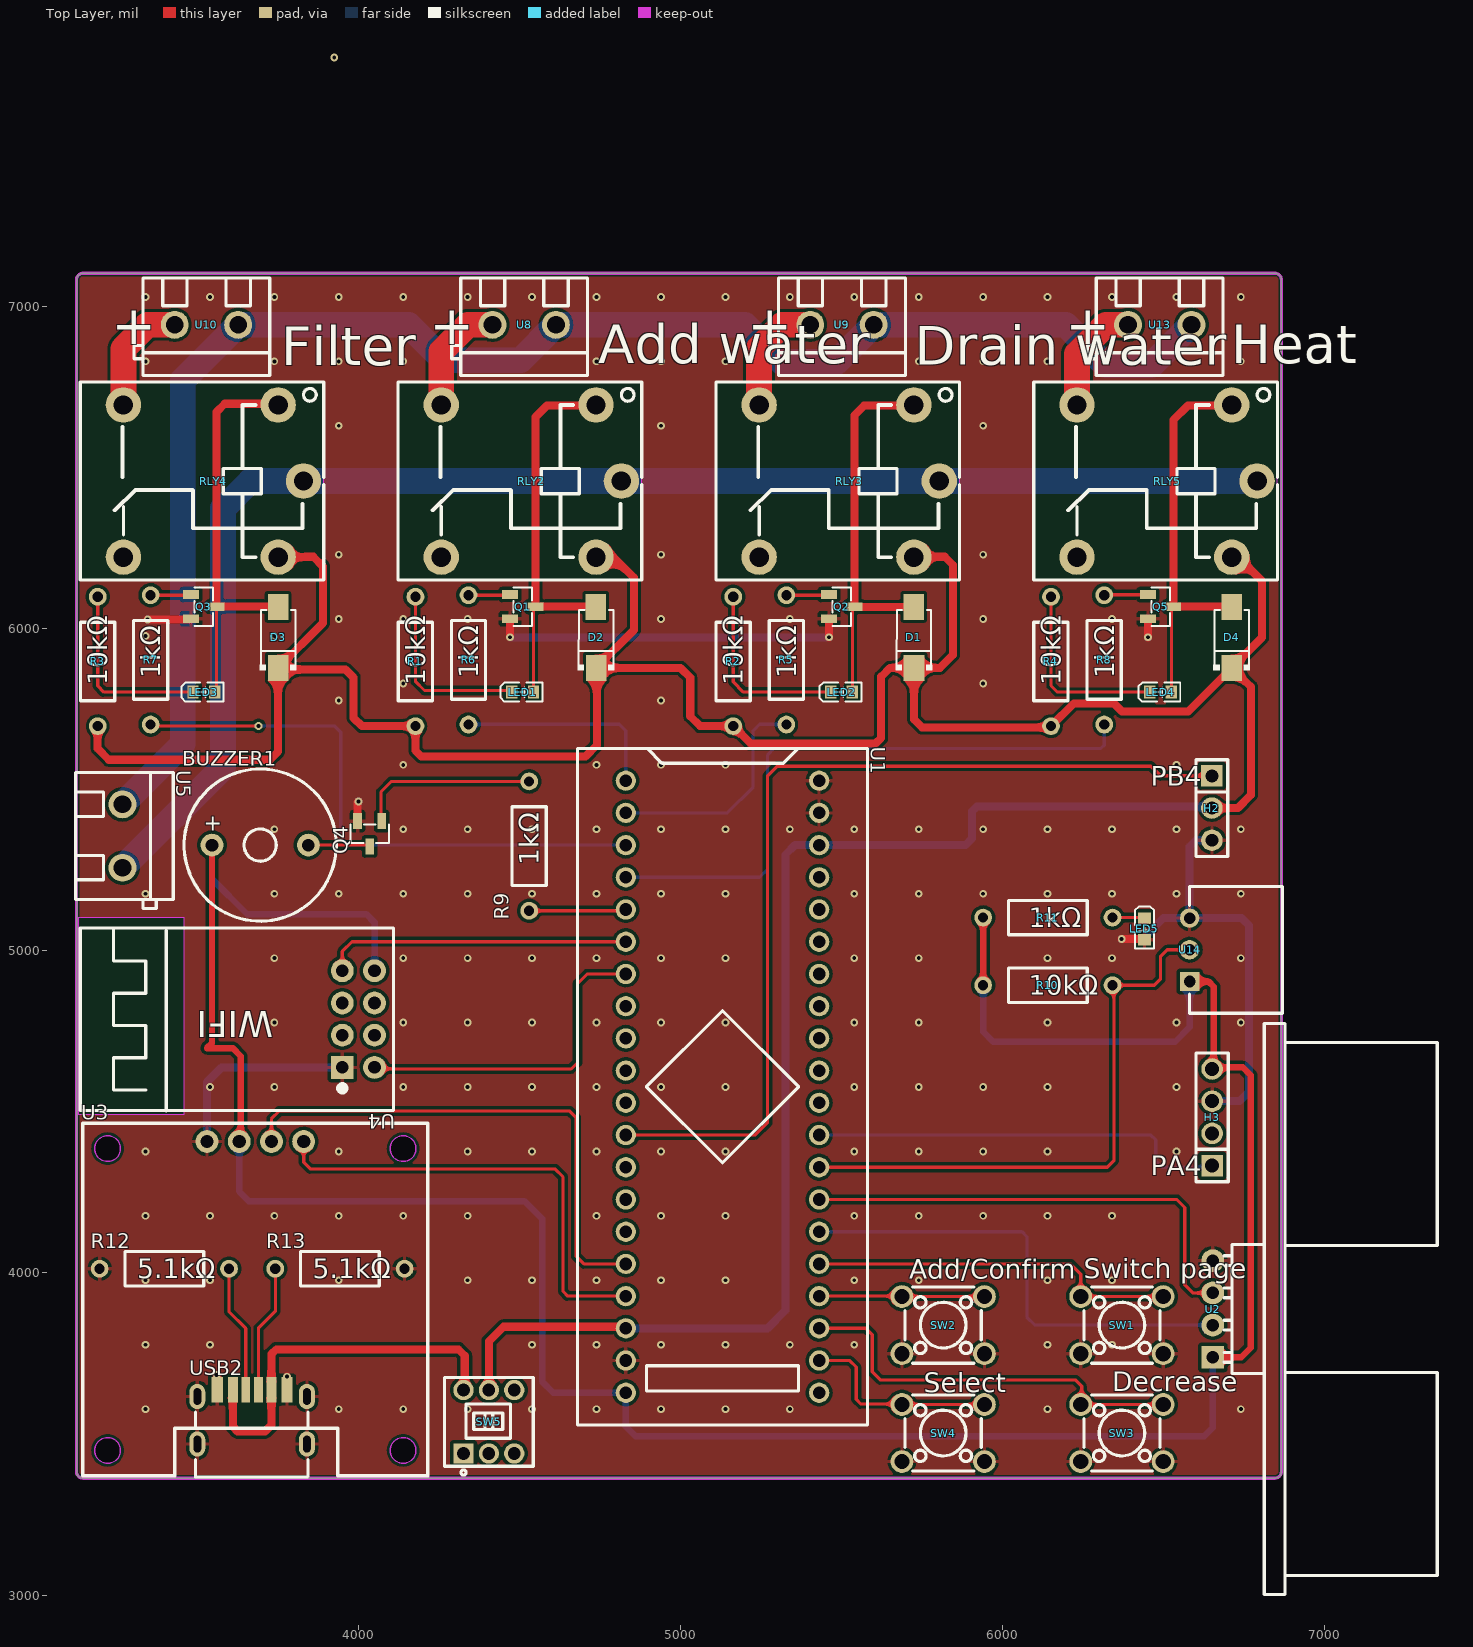
[diagram p0: Top Layer view]
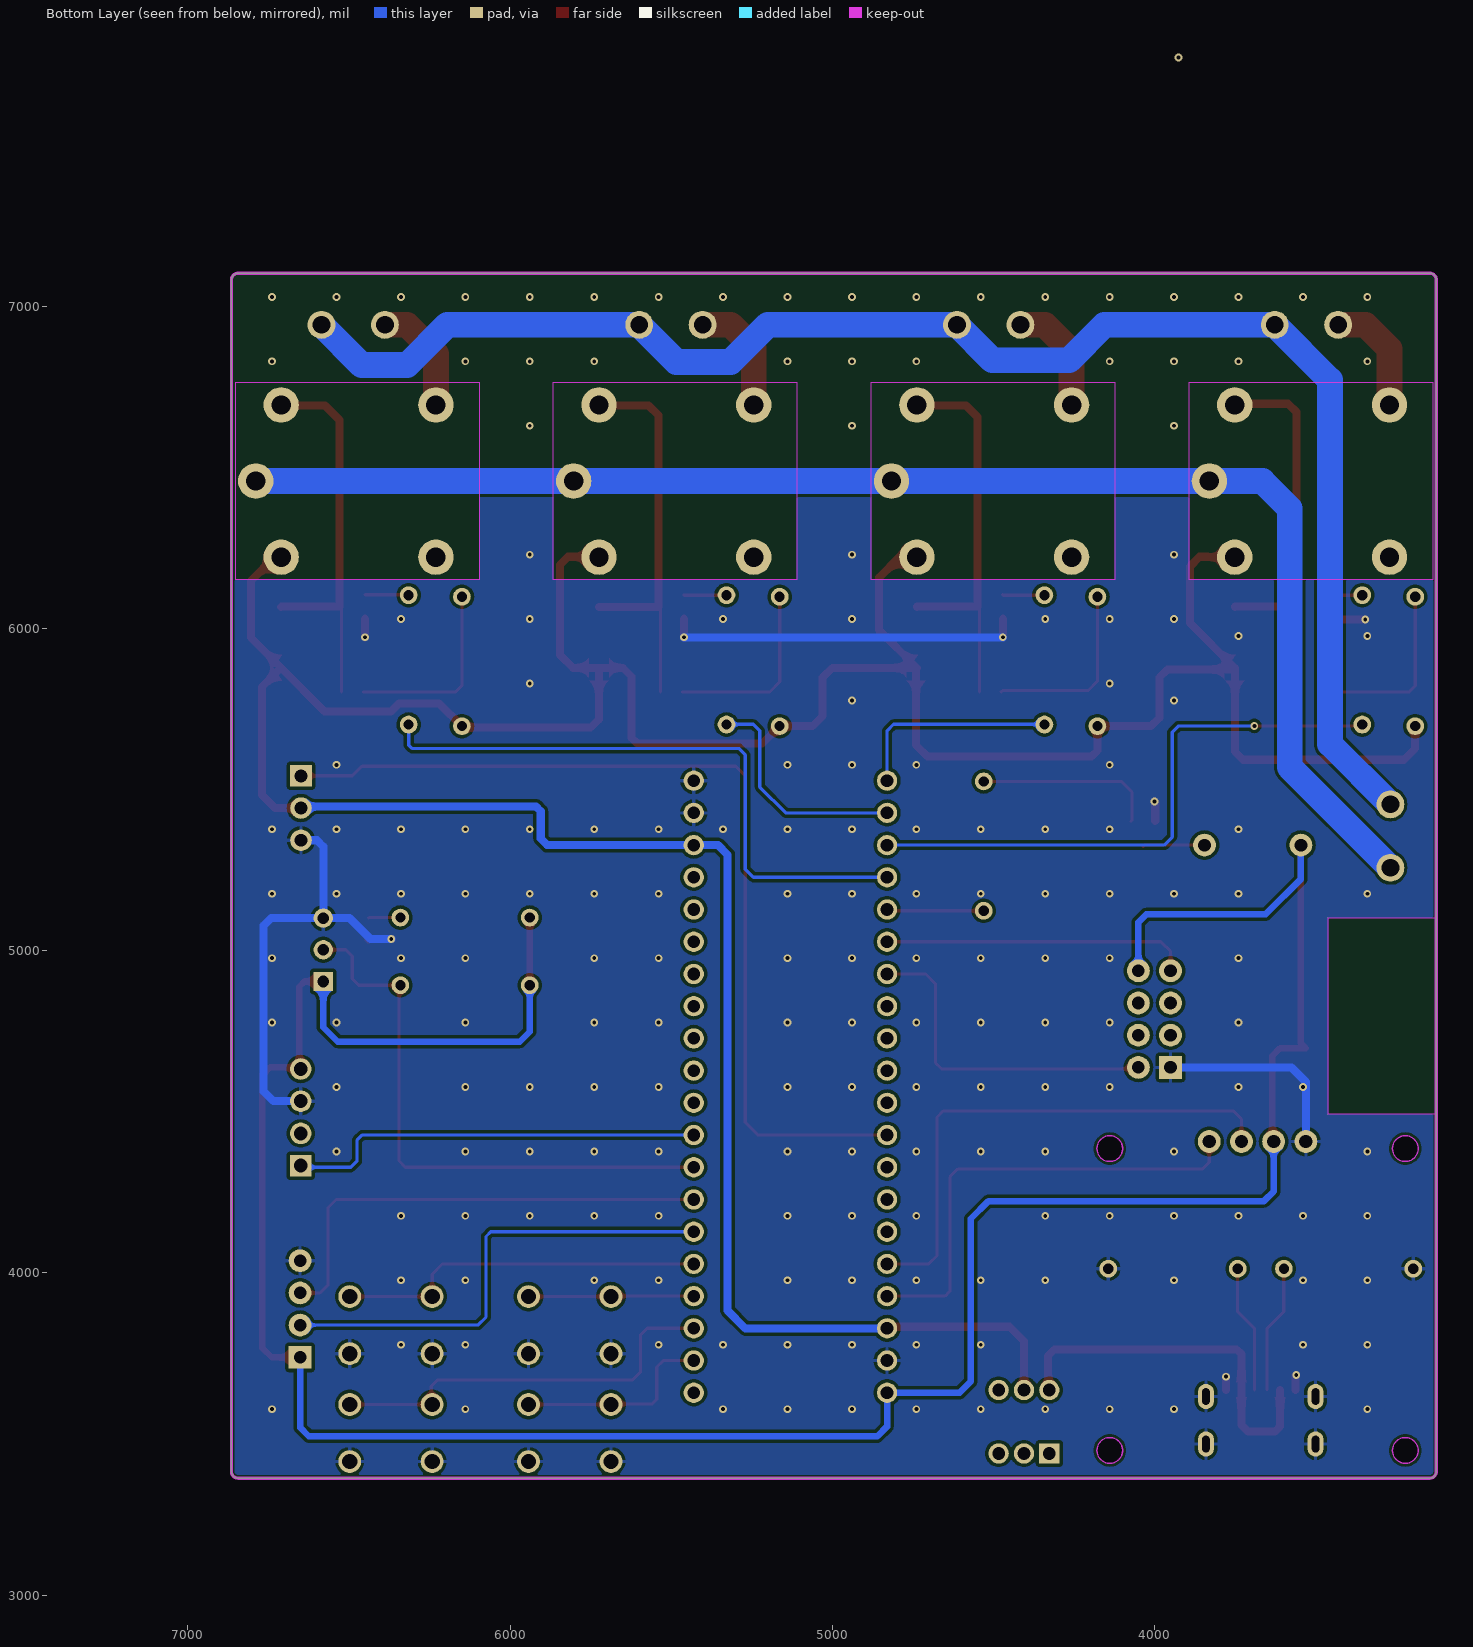
[diagram p1: Bottom Layer view, seen from below]
# Altium PCB MISC62342.pcbdoc (part 1 of 2)
Units mil, origin at the board's own origin, x right, y up, seen from the top; angles counter-clockwise.
Board outline 3740 x 3740 mil, 2 copper layers (Top Layer, Bottom Layer), stack 62.206 mil thick; 50 components, 45 nets, 189 pads, 190 vias.

## Layer stack, top to bottom
Top Solder Mask Layer: solder mask 0.394, Dk 3.3
Top Layer: signal copper 1.379
Dielectric1: surface 59.449, FR4, Dk 4.5
Bottom Layer: signal copper 1.378
Bottom Solder Mask Layer: solder mask 0.394, Dk 3.3

## Board outline
3145,7103.19 ccw(c3145,7083.19) 3125,7083.19 3125,3383.19 ccw(c3145,3383.19) 3145,3363.19 6845,3363.19 ccw(c6845,3383.19) 6865,3383.19 6865,7083.19 ccw(c6845,7083.19) 6845,7103.19

## Design rules (kind name [scope] priority, off if disabled: settings)
BoardOutlineClearance copperThickness2oz_1 [All] p2 off: genericclearance=7.99 ignorepadtopadclearanceinfootprint=FALSE except(0: Arc-SplitContinuation Track-SplitContinuation SMDPad-SplitContinuation THPad-SplitContinuation Via-SplitContinuation Fill-SplitContinuation Region-SplitContinuation Poly-SplitContinuation Text-SplitContinuation Hole-SplitContinuation; 5.98: Arc-CutoutEdge Track-CutoutEdge SMDPad-CutoutEdge THPad-CutoutEdge Via-CutoutEdge Text-CutoutEdge; 6.9: Hole-OutlineEdge Hole-CutoutEdge; 10: Poly-OutlineEdge Poly-CutoutEdge; 11.81: Arc-OutlineEdge Track-OutlineEdge SMDPad-OutlineEdge THPad-OutlineEdge Via-OutlineEdge Fill-OutlineEdge Region-OutlineEdge Text-OutlineEdge Fill-CutoutEdge Region-CutoutEdge)
BoardOutlineClearance Plane_innerPlane_1 [All] p4 off: genericclearance=4.02 ignorepadtopadclearanceinfootprint=FALSE except(0: Arc-SplitContinuation Track-SplitContinuation SMDPad-SplitContinuation THPad-SplitContinuation Via-SplitContinuation Fill-SplitContinuation Region-SplitContinuation Poly-SplitContinuation Text-SplitContinuation Hole-SplitContinuation; 5.98: Arc-CutoutEdge Track-CutoutEdge SMDPad-CutoutEdge THPad-CutoutEdge Via-CutoutEdge Text-CutoutEdge; 6.9: Hole-OutlineEdge Hole-CutoutEdge; 10: Poly-OutlineEdge Poly-CutoutEdge; 11.81: Arc-OutlineEdge Track-OutlineEdge SMDPad-OutlineEdge THPad-OutlineEdge Via-OutlineEdge Fill-OutlineEdge Region-OutlineEdge Text-OutlineEdge Fill-CutoutEdge Region-CutoutEdge)
BoardOutlineClearance Copper_copperRegion_1 [All] p6 off: genericclearance=4.02 ignorepadtopadclearanceinfootprint=FALSE except(0: Arc-SplitContinuation Track-SplitContinuation SMDPad-SplitContinuation THPad-SplitContinuation Via-SplitContinuation Fill-SplitContinuation Region-SplitContinuation Poly-SplitContinuation Text-SplitContinuation Hole-SplitContinuation; 5.98: Arc-CutoutEdge Track-CutoutEdge SMDPad-CutoutEdge THPad-CutoutEdge Via-CutoutEdge Text-CutoutEdge; 6.9: Hole-OutlineEdge Hole-CutoutEdge; 10: Poly-OutlineEdge Poly-CutoutEdge; 11.81: Arc-OutlineEdge Track-OutlineEdge SMDPad-OutlineEdge THPad-OutlineEdge Via-OutlineEdge Fill-OutlineEdge Region-OutlineEdge Text-OutlineEdge Fill-CutoutEdge Region-CutoutEdge)
BoardOutlineClearance copperThickness1oz_1 [All] p8: genericclearance=4.02 ignorepadtopadclearanceinfootprint=FALSE except(0: Arc-SplitContinuation Track-SplitContinuation SMDPad-SplitContinuation THPad-SplitContinuation Via-SplitContinuation Fill-SplitContinuation Region-SplitContinuation Poly-SplitContinuation Text-SplitContinuation Hole-SplitContinuation; 5.98: Arc-CutoutEdge Track-CutoutEdge SMDPad-CutoutEdge THPad-CutoutEdge Via-CutoutEdge Text-CutoutEdge; 6.9: Hole-OutlineEdge Hole-CutoutEdge; 10: Poly-OutlineEdge Poly-CutoutEdge; 11.81: Arc-OutlineEdge Track-OutlineEdge SMDPad-OutlineEdge THPad-OutlineEdge Via-OutlineEdge Fill-OutlineEdge Region-OutlineEdge Text-OutlineEdge Fill-CutoutEdge Region-CutoutEdge)
Clearance copperThickness2oz [All] p1 off: gap=7.99 ignorepadtopadclearanceinfootprint=FALSE except(5.98: SMDPad-Track SMDPad-SMDPad THPad-Track SMDPad-THPad THPad-THPad Track-Via SMDPad-Via THPad-Via Via-Via Fill-SMDPad Region-SMDPad Fill-THPad Region-THPad Fill-Via Region-Via Fill-Fill Fill-Region Region-Region Arc-Track Arc-SMDPad Arc-THPad Arc-Via Fill-Arc Region-Arc Arc-Arc Text-Track SMDPad-Text Text-THPad Text-Via Fill-Text Region-Text Arc-Text Text-Text; 6.9: Hole-Track Hole-SMDPad Hole-THPad Hole-Via Fill-Hole Region-Hole Hole-Arc Hole-Text; 10: Poly-Track Poly-SMDPad Poly-THPad Poly-Via Poly-Fill Poly-Region Poly-Poly Poly-Arc Poly-Text Poly-Hole; 11.81: Fill-Track Region-Track)
Clearance Plane_innerPlane [All] p3 off: gap=4.02 ignorepadtopadclearanceinfootprint=FALSE except(5.98: SMDPad-Track SMDPad-SMDPad THPad-Track SMDPad-THPad THPad-THPad Track-Via SMDPad-Via THPad-Via Via-Via Fill-SMDPad Region-SMDPad Fill-THPad Region-THPad Fill-Via Region-Via Fill-Fill Fill-Region Region-Region Arc-Track Arc-SMDPad Arc-THPad Arc-Via Fill-Arc Region-Arc Arc-Arc Text-Track SMDPad-Text Text-THPad Text-Via Fill-Text Region-Text Arc-Text Text-Text; 6.9: Hole-Track Hole-SMDPad Hole-THPad Hole-Via Fill-Hole Region-Hole Hole-Arc Hole-Text; 10: Poly-Track Poly-SMDPad Poly-THPad Poly-Via Poly-Fill Poly-Region Poly-Poly Poly-Arc Poly-Text Poly-Hole; 11.81: Fill-Track Region-Track)
Clearance Copper_copperRegion [All] p5 off: gap=4.02 ignorepadtopadclearanceinfootprint=FALSE except(5.98: SMDPad-Track SMDPad-SMDPad THPad-Track SMDPad-THPad THPad-THPad Track-Via SMDPad-Via THPad-Via Via-Via Fill-SMDPad Region-SMDPad Fill-THPad Region-THPad Fill-Via Region-Via Fill-Fill Fill-Region Region-Region Arc-Track Arc-SMDPad Arc-THPad Arc-Via Fill-Arc Region-Arc Arc-Arc Text-Track SMDPad-Text Text-THPad Text-Via Fill-Text Region-Text Arc-Text Text-Text; 6.9: Hole-Track Hole-SMDPad Hole-THPad Hole-Via Fill-Hole Region-Hole Hole-Arc Hole-Text; 10: Poly-Track Poly-SMDPad Poly-THPad Poly-Via Poly-Fill Poly-Region Poly-Poly Poly-Arc Poly-Text Poly-Hole; 11.81: Fill-Track Region-Track)
Clearance copperThickness1oz [All] p7: gap=4.02 ignorepadtopadclearanceinfootprint=FALSE except(5.98: SMDPad-Track SMDPad-SMDPad THPad-Track SMDPad-THPad THPad-THPad Track-Via SMDPad-Via THPad-Via Via-Via Fill-SMDPad Region-SMDPad Fill-THPad Region-THPad Fill-Via Region-Via Fill-Fill Fill-Region Region-Region Arc-Track Arc-SMDPad Arc-THPad Arc-Via Fill-Arc Region-Arc Arc-Arc Text-Track SMDPad-Text Text-THPad Text-Via Fill-Text Region-Text Arc-Text Text-Text; 6.9: Hole-Track Hole-SMDPad Hole-THPad Hole-Via Fill-Hole Region-Hole Hole-Arc Hole-Text; 10: Poly-Track Poly-SMDPad Poly-THPad Poly-Via Poly-Fill Poly-Region Poly-Poly Poly-Arc Poly-Text Poly-Hole; 11.81: Fill-Track Region-Track)
DiffPairsRouting differentialPair [All] p1: maxlimit=6 minlimit=6 mostfreqgap=6 toplayer_minwidth=5 toplayer_prefwidth=10 toplayer_maxwidth=100 toplayer_mingap=6 toplayer_prefgap=6 toplayer_maxgap=6 bottomlayer_minwidth=5 bottomlayer_prefwidth=10 bottomlayer_maxwidth=100 bottomlayer_mingap=6 bottomlayer_prefgap=6 bottomlayer_maxgap=6 maxuncoupledlength=10
HoleToHoleClearance otherClearance [All] p1: gap=11.81 allowstackedmicrovias=TRUE
Length netLength [All] p1: minlimit=0 maxlimit=0
PasteMaskExpansion pasteMaskExpansion [All] p1: expansion=0
PlaneConnect innerPlane [All] p1: planeconnectstyle=Relief reliefexpansion=20 reliefentries=4 reliefconductorwidth=10 reliefairgap=10
PolygonConnect copperRegion [All] p1: connectstyle=Relief reliefconductorwidth=10 reliefentries=4 polygonreliefangle="90 Angle" airgapwidth=10 via.connectstyle=Relief via.reliefconductorwidth=10 via.reliefentries=4 via.polygonreliefangle="90 Angle" via.airgapwidth=10
RoutingVias viaSize [All] p1: holewidth=12.01 width=24.02 viastyle="Through Hole" minholewidth=11.81 minwidth=19.68 maxholewidth=248.03 maxwidth=393.7
SolderMaskExpansion solderMaskExpansion [IsVia] p1: expansion=-1000 istentingtop=TRUE
SolderMaskExpansion solderMaskExpansion [All] p2: expansion=2 istentingtop=FALSE
Width copperThickness2oz_2 [All] p1 off: maxlimit=100 minlimit=8 preferedwidth=10
Width copperThickness1oz_2 [All] p2: maxlimit=100 minlimit=5 preferedwidth=10

## Components (designator, comment, footprint, x,y, rotation, side; value= is the part's Value field where it differs from the comment)
BUZZER1 "2.4kHz" BUZ-TH_BD12.0-P7.60-D0.6-FD 3695,5328.19 r0 top
D1 "1N4007A-AAF" SMA_L4.3-W2.6-LS5.0-RD 5724.12,5973.19 r90 top
D2 "1N4007A-AAF" SMA_L4.3-W2.6-LS5.0-RD 4737.46,5973.19 r90 top
D3 "1N4007A-AAF" SMA_L4.3-W2.6-LS5.0-RD 3750.79,5973.19 r90 top
D4 "1N4007A-AAF" SMA_L4.3-W2.6-LS5.0-RD 6710.79,5973.19 r90 top
H2 "PZ254V-11-03P" HDR-TH_3P-P2.54-V-M_PZ254V-11-03P 6649.21,5443.19 r270 top
H3 "PZ254V-11-04P" HDR-TH_4P-P2.54-V-M 6650,4483.19 r90 top
LED1 "GL0603UR01" LED0603-FD 4510,5803.19 r180 top
LED2 "GL0603UR01" LED0603-FD 5500,5803.19 r180 top
LED3 "GL0603UR01" LED0603-FD 3520,5803.19 r180 top
LED4 "GL0603UR01" LED0603-FD 6490,5803.19 r180 top
LED5 "GL0603UR01" LED0603-FD 6440,5068.19 r90 top
Q1 "SS8050" SOT-23-3_L2.9-W1.3-P1.90-LS2.4-BR 4510,6068.19 r180 top
Q2 "SS8050" SOT-23-3_L2.9-W1.3-P1.90-LS2.4-BR 5500,6068.19 r180 top
Q3 "SS8050" SOT-23-3_L2.9-W1.3-P1.90-LS2.4-BR 3520,6068.19 r180 top
Q4 "SS8050" SOT-23-3_L2.9-W1.3-P1.90-LS2.4-BR 4035,5363.19 r90 top
Q5 "SS8050" SOT-23-3_L2.9-W1.3-P1.90-LS2.4-BR 6490,6068.19 r180 top
R1 "10kΩ" RES-TH_BD2.7-L6.2-P10.20-D0.4 4177.02,5898.19 r270 top
R2 "10kΩ" RES-TH_BD2.7-L6.2-P10.20-D0.4 5163.37,5898.19 r270 top
R3 "10kΩ" RES-TH_BD2.7-L6.2-P10.20-D0.4 3190.66,5898.19 r270 top
R4 "10kΩ" RES-TH_BD2.7-L6.2-P10.20-D0.4 6149.72,5898.19 r270 top
R5 "1kΩ" RES-TH_BD2.7-L6.2-P10.20-D0.4 5328.33,5903.19 r90 top
R6 "1kΩ" RES-TH_BD2.7-L6.2-P10.20-D0.4 4341.67,5903.19 r90 top
R7 "1kΩ" RES-TH_BD2.7-L6.2-P10.20-D0.4 3355,5903.19 r90 top
R8 "1kΩ" RES-TH_BD2.7-L6.2-P10.20-D0.4 6315,5903.19 r90 top
R9 "1kΩ" RES-TH_BD2.7-L6.2-P10.20-D0.4 4530,5325.04 r90 top
R10 "10kΩ" RES-TH_BD2.7-L6.2-P10.20-D0.4 6140,4893.19 r180 top
R11 "1kΩ" RES-TH_BD2.7-L6.2-P10.20-D0.4 6140,5103.19 r180 top
R12 "5.1kΩ" RES-TH_BD2.7-L6.2-P10.20-D0.4 3397.56,4013.19 r0 top
R13 "5.1kΩ" RES-TH_BD2.7-L6.2-P10.20-D0.4 3942.44,4013.19 r0 top
RLY2 "SRD-05VDC-SL-C" RELAY-TH_SRD-XXVDC-XL-C 4536.67,6458.19 r180 top
RLY3 "SRD-05VDC-SL-C" RELAY-TH_SRD-XXVDC-XL-C 5523.33,6458.19 r180 top
RLY4 "SRD-05VDC-SL-C" RELAY-TH_SRD-XXVDC-XL-C 3550,6458.19 r180 top
RLY5 "SRD-05VDC-SL-C" RELAY-TH_SRD-XXVDC-XL-C 6510,6458.19 r180 top
SW1 "TS665CJ" SW-TH_4P-L6.0-W6.0-P4.50-LS6.5 6370,3838.19 r0 top
SW2 "TS665CJ" SW-TH_4P-L6.0-W6.0-P4.50-LS6.5 5815,3838.19 r0 top
SW3 "TS665CJ" SW-TH_4P-L6.0-W6.0-P4.50-LS6.5 6370,3503.19 r0 top
SW4 "TS665CJ" SW-TH_4P-L6.0-W6.0-P4.50-LS6.5 5815,3503.19 r0 top
SW5 "TK-6700-1" SW-TH_TK-6700-1 4405,3538.19 r0 top
U1 "LCKFB-DKX-STM32F103C8T6" CONN-TH_L53.3-W22.9_STM32F103C8T6-CARD 5130,4578.19 r270 top
U2 "HC-SR04" TH_HC-SR04V 6651.97,3888.19 r90 top
U3 "HS96L03W2C03" OLED-TH_L27.8-W27.2-P2.54_C9900033791 3680,4408.19 r0 top
U4 "2.4GHz" WIFIM-TH_8P-L24.7-W14.4-P2.54 4000,4788.19 r180 top
U5 "KF301-5.0-2P" CONN-TH_P5.00_KF301-5.0-2P 3267.64,5356.28 r270 top
U8 "KF301-5.0-2P" CONN-TH_P5.00_KF301-5.0-2P 4514.53,6943.19 r180 top
U9 "KF301-5.0-2P" CONN-TH_P5.00_KF301-5.0-2P 5500.88,6943.19 r180 top
U10 "KF301-5.0-2P" CONN-TH_P5.00_KF301-5.0-2P 3528.18,6943.19 r180 top
U13 "KF301-5.0-2P" CONN-TH_P5.00_KF301-5.0-2P 6487.23,6943.19 r180 top
U14 "WAFER-XH2.54-3PWZ" CONN-TH_3P-P2.50_WAFER-XH2.54-3PWZ 6580,5003.19 r90 top
USB2 "" "USB_ TYPE-C-6P" 3665,3553.19 r0 top

## Footprints (in the part's own frame and the unit in brackets; to place one, negate y for a bottom-side part, rotate by r counter-clockwise, add the part's x,y. Pads: shape width x height; smd on the part's side, far side on the other; paste and mask are expansions set on the pad)
BUZ-TH_BD12.0-P7.60-D0.6-FD [mm]
  round 1.8 hole 1: 1(-3.8,0) 2(3.8,0)
  silkscreen extent -6,-6 6,6
CONN-TH_3P-P2.50_WAFER-XH2.54-3PWZ [mil]
  rect 60x60 hole 36 paste+0 mask+1.97: 1(-98.43,0)
  round 60 hole 36 paste+0 mask+1.97: 2(-0.01,0) 3(98.42,0)
  silkscreen extent -197,-288 197,0
CONN-TH_L53.3-W22.9_STM32F103C8T6-CARD [mm]
  round 1.6 hole 1: 1(-24.13,-7.62) 2(-21.59,-7.62) 3(-19.05,-7.62) 4(-16.51,-7.62) 5(-13.97,-7.62) 6(-11.43,-7.62) 7(-8.89,-7.62) 8(-6.35,-7.62) 9(-3.81,-7.62) 10(-1.27,-7.62) 11(1.27,-7.62) 12(3.81,-7.62) 13(6.35,-7.62) 14(8.89,-7.62) 15(11.43,-7.62) 16(13.97,-7.62) 17(16.51,-7.62) 18(19.05,-7.62) 19(21.59,-7.62) 20(24.13,-7.62) 21(24.13,7.62) 22(21.59,7.62) 23(19.05,7.62) 24(16.51,7.62) 25(13.97,7.62) 26(11.43,7.62) 27(8.89,7.62) 28(6.35,7.62) 29(3.81,7.62) 30(1.27,7.62) 31(-1.27,7.62) 32(-3.81,7.62) 33(-6.35,7.62) 34(-8.89,7.62) 35(-11.43,7.62) 36(-13.97,7.62) 37(-16.51,7.62) 38(-19.05,7.62) 39(-21.59,7.62) 40(-24.13,7.62)
  silkscreen extent -26.67,-11.43 26.67,11.43
CONN-TH_P5.00_KF301-5.0-2P [mm]
  round 2.2 hole 1.4 paste+0 mask+0.05: 1(-2.5,0) 2(2.5,0)
  silkscreen extent -5,-3.7 5.71,4
HDR-TH_3P-P2.54-V-M_PZ254V-11-03P [mm]
  rect 1.7x1.7 hole 1.02: 1(-2.54,0)
  round 1.7 hole 1.02: 2(0,0) 3(2.54,0)
  silkscreen extent -3.81,-1.25 3.81,1.25
HDR-TH_4P-P2.54-V-M [mm]
  rect 1.7x1.7 hole 1.1: 1(-3.81,0)
  round 1.7 hole 1.1: 2(-1.27,0) 3(1.27,0) 4(3.81,0)
  silkscreen extent -5.08,-1.27 5.08,1.27
LED0603-FD [mm]
  rect 0.9x1 smd: 1(-0.85,0) 2(0.85,0)
  silkscreen extent -1.55,-0.75 1.75,0.75
OLED-TH_L27.8-W27.2-P2.54_C9900033791 [mm]
  round 1.8 hole 1.05 paste+0 mask+0.05: 1(-3.81,0) 2(-1.27,0) 3(1.27,0) 4(3.81,0)
  Board Outline Layer circle w0.003: c-11.65,-0.56 r1.016
  Board Outline Layer circle w0.003: c11.65,-0.56 r1.016
  Board Outline Layer circle w0.003: c-11.65,-24.36 r1.016
  Board Outline Layer circle w0.003: c11.65,-24.36 r1.016
  Board Outline Layer region: -10.634,-0.56 -10.735,-1.001 -11.016,-1.354 -11.424,-1.551 -11.876,-1.551 -12.283,-1.354 -12.565,-1.001 -12.666,-0.56 -12.666,-0.56 -12.565,-0.119 -12.283,0.234 -11.876,0.431 -11.424,0.431 -11.016,0.234 -10.735,-0.119 -10.634,-0.56
  Board Outline Layer region: -10.634,-0.56 -10.643,-0.698 -10.672,-0.834 -10.718,-0.965 -10.782,-1.088 -10.862,-1.201 -10.956,-1.303 -11.064,-1.39 -11.183,-1.462 -11.31,-1.517 -11.443,-1.555 -11.581,-1.574 -11.719,-1.574 -11.857,-1.555 -11.99,-1.517 -12.117,-1.462 -12.236,-1.39 -12.343,-1.303 -12.438,-1.201 -12.518,-1.088 -12.582,-0.965 -12.628,-0.834 -12.656,-0.698 -12.666,-0.56 -12.656,-0.422 -12.628,-0.286 -12.582,-0.155 -12.518,-0.032 -12.438,0.081 -12.343,0.183 -12.236,0.27 -12.117,0.342 -11.99,0.397 -11.857,0.435 -11.719,0.454 -11.581,0.454 -11.443,0.435 -11.31,0.397 -11.183,0.342 -11.064,0.27 -10.956,0.183 -10.862,0.081 -10.782,-0.032 -10.718,-0.155 -10.672,-0.286 -10.643,-0.422
  Board Outline Layer region: 12.666,-0.56 12.565,-1.001 12.283,-1.354 11.876,-1.551 11.424,-1.551 11.017,-1.354 10.735,-1.001 10.634,-0.56 10.634,-0.56 10.735,-0.119 11.017,0.234 11.424,0.431 11.876,0.431 12.283,0.234 12.565,-0.119 12.666,-0.56
  Board Outline Layer region: 12.666,-0.56 12.657,-0.698 12.628,-0.834 12.582,-0.965 12.518,-1.088 12.438,-1.201 12.343,-1.303 12.236,-1.39 12.117,-1.462 11.99,-1.517 11.857,-1.555 11.719,-1.574 11.581,-1.574 11.443,-1.555 11.31,-1.517 11.183,-1.462 11.064,-1.39 10.957,-1.303 10.862,-1.201 10.782,-1.088 10.718,-0.965 10.672,-0.834 10.643,-0.698 10.634,-0.56 10.643,-0.422 10.672,-0.286 10.718,-0.155 10.782,-0.032 10.862,0.081 10.957,0.183 11.064,0.27 11.183,0.342 11.31,0.397 11.443,0.435 11.581,0.454 11.719,0.454 11.857,0.435 11.99,0.397 12.117,0.342 12.236,0.27 12.343,0.183 12.438,0.081 12.518,-0.032 12.582,-0.155 12.628,-0.286 12.657,-0.422
  Board Outline Layer region: -10.634,-24.36 -10.735,-24.801 -11.016,-25.154 -11.424,-25.35 -11.876,-25.35 -12.283,-25.154 -12.565,-24.801 -12.666,-24.36 -12.666,-24.36 -12.565,-23.919 -12.283,-23.566 -11.876,-23.369 -11.424,-23.369 -11.016,-23.566 -10.735,-23.919 -10.634,-24.36
  Board Outline Layer region: -10.634,-24.36 -10.643,-24.498 -10.672,-24.634 -10.718,-24.765 -10.782,-24.888 -10.862,-25.001 -10.956,-25.102 -11.064,-25.19 -11.183,-25.262 -11.31,-25.317 -11.443,-25.355 -11.581,-25.374 -11.719,-25.374 -11.857,-25.355 -11.99,-25.317 -12.117,-25.262 -12.236,-25.19 -12.343,-25.102 -12.438,-25.001 -12.518,-24.888 -12.582,-24.765 -12.628,-24.634 -12.656,-24.498 -12.666,-24.36 -12.656,-24.222 -12.628,-24.086 -12.582,-23.955 -12.518,-23.832 -12.438,-23.719 -12.343,-23.617 -12.236,-23.53 -12.117,-23.458 -11.99,-23.403 -11.857,-23.365 -11.719,-23.346 -11.581,-23.346 -11.443,-23.365 -11.31,-23.403 -11.183,-23.458 -11.064,-23.53 -10.956,-23.617 -10.862,-23.719 -10.782,-23.832 -10.718,-23.955 -10.672,-24.086 -10.643,-24.222
  Board Outline Layer region: 12.666,-24.36 12.565,-24.801 12.283,-25.154 11.876,-25.35 11.424,-25.35 11.017,-25.154 10.735,-24.801 10.634,-24.36 10.634,-24.36 10.735,-23.919 11.017,-23.566 11.424,-23.369 11.876,-23.369 12.283,-23.566 12.565,-23.919 12.666,-24.36
  Board Outline Layer region: 12.666,-24.36 12.657,-24.498 12.628,-24.634 12.582,-24.765 12.518,-24.888 12.438,-25.001 12.343,-25.102 12.236,-25.19 12.117,-25.262 11.99,-25.317 11.857,-25.355 11.719,-25.374 11.581,-25.374 11.443,-25.355 11.31,-25.317 11.183,-25.262 11.064,-25.19 10.957,-25.102 10.862,-25.001 10.782,-24.888 10.718,-24.765 10.672,-24.634 10.643,-24.498 10.634,-24.36 10.643,-24.222 10.672,-24.086 10.718,-23.955 10.782,-23.832 10.862,-23.719 10.957,-23.617 11.064,-23.53 11.183,-23.458 11.31,-23.403 11.443,-23.365 11.581,-23.346 11.719,-23.346 11.857,-23.365 11.99,-23.403 12.117,-23.458 12.236,-23.53 12.343,-23.617 12.438,-23.719 12.518,-23.832 12.582,-23.955 12.628,-24.086 12.657,-24.222
  Multi-Layer board cut-out: -10.634,-0.56 -10.735,-1.001 -11.016,-1.354 -11.424,-1.551 -11.876,-1.551 -12.283,-1.354 -12.565,-1.001 -12.666,-0.56 -12.666,-0.56 -12.565,-0.119 -12.283,0.234 -11.876,0.431 -11.424,0.431 -11.016,0.234 -10.735,-0.119 -10.634,-0.56
  Multi-Layer board cut-out: 12.666,-0.56 12.565,-1.001 12.283,-1.354 11.876,-1.551 11.424,-1.551 11.017,-1.354 10.735,-1.001 10.634,-0.56 10.634,-0.56 10.735,-0.119 11.017,0.234 11.424,0.431 11.876,0.431 12.283,0.234 12.565,-0.119 12.666,-0.56
  Multi-Layer board cut-out: -10.634,-24.36 -10.735,-24.801 -11.016,-25.154 -11.424,-25.35 -11.876,-25.35 -12.283,-25.154 -12.565,-24.801 -12.666,-24.36 -12.666,-24.36 -12.565,-23.919 -12.283,-23.566 -11.876,-23.369 -11.424,-23.369 -11.016,-23.566 -10.735,-23.919 -10.634,-24.36
  Multi-Layer board cut-out: 12.666,-24.36 12.565,-24.801 12.283,-25.154 11.876,-25.35 11.424,-25.35 11.017,-25.154 10.735,-24.801 10.634,-24.36 10.634,-24.36 10.735,-23.919 11.017,-23.566 11.424,-23.369 11.876,-23.369 12.283,-23.566 12.565,-23.919 12.666,-24.36
  silkscreen extent -13.6,-26.36 13.6,1.44
RELAY-TH_SRD-XXVDC-XL-C [mil]
  round 110 hole 60: 1(-200.79,-236.22) 2(279.52,-236.2) 3(279.53,236.2) 4(-200.79,236.22) 5(-279.53,0)
  silkscreen extent -342,-307 413,307
RES-TH_BD2.7-L6.2-P10.20-D0.4 [mm]
  round 1.4 hole 0.8 copper offset 0,0: 1(-5.1,0) 2(5.1,0)
  silkscreen extent -3.1,-1.35 3.1,1.35
SMA_L4.3-W2.6-LS5.0-RD [mm]
  rect 2.046x1.62 smd: 1(-2.404,-0.009) 2(2.404,0.009)
  silkscreen extent -2.61,-1.44 2.16,1.44
SOT-23-3_L2.9-W1.3-P1.90-LS2.4-BR [mm]
  rect 1.25x0.7 smd: 1(1,-0.95) 2(1,0.95) 3(-1,0)
  silkscreen extent -0.73,-1.53 0.73,1.53
SW-TH_4P-L6.0-W6.0-P4.50-LS6.5 [mm]
  round 1.8 hole 1.2: 1(-3.25,2.25) 2(3.25,2.25) 3(-3.25,-2.25) 4(3.25,-2.25)
  silkscreen extent -3,-3 3,3
SW-TH_TK-6700-1 [mm]
  rect 1.6x1.6 hole 1: 1(-2,-2.5)
  round 1.6 hole 1: 2(0,-2.5) 3(2,-2.5)
  round 1.6 hole 1 copper offset 0,0: 4(-2,2.5) 5(0,2.5) 6(2,2.5)
  silkscreen extent -3.5,-4.2 3.5,3.5
TH_HC-SR04V [mm]
  rect 1.8x1.8 hole 1.001: 1(-3.81,0)
  round 1.8 hole 1.001: 2(-1.27,0) 3(1.27,0) 4(3.81,0)
  silkscreen extent -22.5,-17.7 22.5,-0.89
"USB_ TYPE-C-6P" [mm]
  oval 1.25x2 hole 0.6 slot 1.3 at 90 deg paste+0 mask+0.05: 7(-4.193,1.611) 8(4.447,1.611) 9(-4.193,-2.139) 10(4.447,-2.139)
  rect 0.7x2.032 smd paste-100 mask+0.05: A5(-0.373,2.139) B5(0.627,2.139)
  rect 0.8x2.032 smd paste-100 mask+0.05: A9(1.647,2.139) B9(-1.393,2.139)
  rect 0.9x2.032 smd paste-100 mask+0.05: A12(2.877,2.139) B12(-2.623,2.139)
  silkscreen extent -4.34,-4.75 4.52,0.39
WIFIM-TH_8P-L24.7-W14.4-P2.54 [mm]
  rect 1.8x1.8 hole 1 paste+0 mask+0.05: 1(1.27,3.81)
  round 1.8 hole 1 paste+0 mask+0.05: 2(1.27,1.27) 3(1.27,-1.27) 4(1.27,-3.81) 5(-1.27,3.81) 6(-1.27,1.27) 7(-1.27,-1.27) 8(-1.27,-3.81)
  silkscreen extent -2.77,-7.19 21.93,7.24

## Via types
v1: diameter 24.02, hole 12, Top Layer to Bottom Layer, 190 vias

## Nets (pads, with @x,y where several pads share a name; then routed paths per layer and width w, separated by ;. In a path a pad name is that pad's centre, name@x,y a point inside that pad or via, vN(x,y) a via of type N, cw(c..) or ccw(c..) an arc to the next point about the centre after c; other vN are vias at no path point)
$1N3766: LED5.2 R11.1 | length 99.8
  Top Layer w10: R11.1@6340.78,5103.19 6438.47,5103.19 LED5.2@6440,5101.65
$1N3772: R12.2 USB2.A5 | length 397.3
  Top Layer w10: R12.2@3598.34,4013.19 3598.35,3879.84 3650.32,3827.87 USB2.A5@3650.32,3637.4
$1N3773: R13.1 USB2.B5 | length 397.9
  Top Layer w10: USB2.B5@3689.69,3637.4 3689.69,3828.19 3742.34,3880.84 3742.34,4012.49 R13.1@3741.66,4013.19
$1N3775: LED3.2 R3.1 | length 580.3
  Top Layer w10: R3.1@3190.66,6098.97 3190.66,5822.52 3210,5803.19 LED3.2@3486.53,5803.19
$1N3776: RLY4.2 U10.2 | length 364.4
  Top Layer w80: RLY4.2@3270.47,6694.39 3270.47,6868.66 3345,6943.19 U10.2@3429.75,6943.19
$1N3777: D3.2 LED3.1 Q3.3 RLY4.1 | length 1266.6
  Top Layer w10: LED3.1@3553.47,5803.19 3559.37,5809.09 Q3.3@3559.37,6068.19
  Top Layer w25: D3.2@3750.42,6067.83 3750.06,6068.19 Q3.3@3559.37,6068.19 3559.37,6672.56 3585,6698.19 3747.01,6698.19 RLY4.1@3750.79,6694.41
$1N3781: Q3.1 R7.2 | length 126.3
  Top Layer w10: R7.2@3355,6103.97 3479.02,6103.98 Q3.1@3480.63,6105.59
$1N3789: D1.2 LED2.1 Q2.3 RLY3.1 | length 1244.3
  Top Layer w10: LED2.1@5533.47,5803.19 5533.47,6062.28 Q2.3@5539.37,6068.19
  Top Layer w25: D1.2@5723.75,6067.83 5539.73,6067.83 Q2.3@5539.37,6068.19 5539.37,6662.56 5570,6693.19 5722.9,6693.19 RLY3.1@5724.12,6694.41
$1N3792: LED4.2 R4.1 | length 590.7
  Top Layer w10: R4.1@6149.72,6098.97 6149.72,5823.47 6170,5803.19 LED4.2@6456.53,5803.19
$1N3795: RLY5.2 U13.2 | length 354.7
  Top Layer w80: RLY5.2@6230.48,6694.39 6230.47,6853.66 6320,6943.19 U13.2@6388.81,6943.19
$1N3797: D4.2 LED4.1 Q5.3 RLY5.1 | length 1228.8
  Top Layer w10: LED4.1@6523.47,5803.19 6523.47,6062.28 Q5.3@6529.37,6068.19
  Top Layer w25: D4.2@6710.42,6067.83 6710.06,6068.19 Q5.3@6529.37,6068.19 6529.37,6647.56 6575,6693.19 6709.57,6693.19 RLY5.1@6710.79,6694.41
$1N3798: Q5.1 R8.2 | length 136.3
  Top Layer w10: R8.2@6315,6103.97 6316.61,6105.59 Q5.1@6450.63,6105.59
$1N3802: Q4.1 R9.2 | length 565.1
  Top Layer w10: Q4.1@4072.4,5402.56 4070,5404.96 4070,5493.19 4102.64,5525.83 R9.2@4530,5525.82
$1N3804: BUZZER1.2 Q4.3 | length 192.2
  Top Layer w10: BUZZER1.2@3844.61,5328.19 4030.63,5328.19 Q4.3@4035,5323.82
$1N3806: LED2.2 R2.1 | length 580.4
  Top Layer w10: R2.1@5163.37,6098.97 5163.37,5834.82 5195,5803.19 LED2.2@5466.53,5803.19
$1N3807: LED1.2 R1.1 | length 576
  Top Layer w10: R1.1@4177.02,6098.97 4177.02,5836.17 4205,5808.19 4471.53,5808.19 LED1.2@4476.53,5803.19
$1N3808: D2.2 LED1.1 Q1.3 RLY2.1 | length 1248
  Top Layer w10: LED1.1@4543.47,5803.19 4543.47,6062.28 Q1.3@4549.37,6068.19
  Top Layer w25: D2.2@4737.09,6067.83 4736.73,6068.19 Q1.3@4549.37,6068.19 4549.37,6657.56 4585,6693.19 4736.24,6693.19 RLY2.1@4737.45,6694.41
$1N3809: RLY2.2 U8.2 | length 359.2
  Top Layer w80: RLY2.2@4257.14,6694.39 4257.14,6860.32 4340,6943.19 U8.2@4416.1,6943.19
$1N3815: RLY3.2 U9.2 | length 365.7
  Top Layer w80: RLY3.2@5243.81,6694.39 5243.8,6871.99 5315,6943.19 U9.2@5402.46,6943.19
$1N3818: Q2.1 R5.2 | length 133
  Top Layer w10: R5.2@5328.33,6103.97 5459.02,6103.98 Q2.1@5460.63,6105.59
$1N3819: Q1.1 R6.2 | length 129.6
  Top Layer w10: R6.2@4341.67,6103.97 4469.02,6103.98 Q1.1@4470.63,6105.59
+3.3V: BUZZER1.1 H3.4 R10.2 R11.2 U1.20 U2.1 U3.2 U4.8 U14.1 | length 8524.7
  Top Layer w20: BUZZER1.1@3545.39,5328.19 3545.39,4713.58 3530,4698.19 3610,4698.19 3635,4673.19 3635,4413.19 U3.2@3630,4408.19 ; R11.2@5929.21,5103.19 5939.21,5093.19 R10.2@5939.22,4893.19 ; U14.1@6580,4904.76 6638.43,4904.76 6655,4888.19 H3.4@6655,4638.19 ; H3.4@6650,4633.19 H3.4@6655,4638.19 ; U2.1@6651.97,3738.19 6740,3738.19 6770,3768.19 6770,4613.19 6745,4638.19 H3.4@6655,4638.19
  Bottom Layer w20: BUZZER1.1@3545.39,5328.19 3545.39,5222.79 3655,5113.19 4025,5113.19 4050,5088.19 U4.8@4050,4938.19 ; U3.2@3630,4408.19 3630,4253.19 3660,4223.19 4515,4223.19 4570,4168.19 4570,3663.19 4605,3628.18 U1.20@4830,3628.19 4830,3523.19 4860,3493.19 6625,3493.19 6651.97,3520.16 U2.1@6651.97,3738.19 ; R10.2@5939.22,4893.19 5939.21,4748.98 5970,4718.19 6535,4718.19 6580,4763.19 U14.1@6580,4904.76
+5V: D1.1 D2.1 D3.1 D4.1 H2.2 R1.2 R2.2 R3.2 R4.2 RLY2.4 RLY3.4 RLY4.4 RLY5.4 SW5.5 U1.18 U1.38 | length 11511.7
  Top Layer w25: R3.2@3190.66,5697.41 3190.66,5627.52 3225,5593.19 3725,5593.19 3750,5618.19 3750,5877.38 D3.1@3751.16,5878.54 ; RLY4.4@3750.79,6221.97 3833.78,6221.97 3835,6223.19 3860,6223.19 3890,6193.19 3890,6017.38 D3.1@3751.16,5878.54 ; SW5.5@4405,3636.62 4405,3788.19 4450,3833.19 4825,3833.19 U1.18@4830,3828.19 ; RLY2.4@4737.45,6221.97 4791.22,6221.97 4855,6158.19 4855,5995.72 D2.1@4737.83,5878.54 ; RLY3.4@5724.12,6221.97 5725.34,6223.19 5820,6223.19 5845,6198.19 5845,5918.19 5805.35,5878.54 D1.1@5724.49,5878.54 ; H2.2@6649.21,5443.19 6730,5443.19 6770,5483.19 6770,5819.7 D4.1@6711.16,5878.54 ; RLY5.4@6710.79,6221.97 6731.22,6221.97 6805,6148.19 6805,5972.38 D4.1@6711.16,5878.54 ; D3.1@3751.16,5878.54 3756.51,5873.19 3960,5873.19 3985,5848.19 3985,5723.19 4010.79,5697.4 R1.2@4177.02,5697.41 4177.02,5621.17 4195,5603.19 4705,5603.19 4740,5638.19 4740,5876.37 4738.18,5878.19 5000,5878.19 5030,5848.19 5030,5728.19 5060.79,5697.4 R2.2@5163.37,5697.41 5217.58,5643.19 5605,5643.19 5622.68,5660.86 5622.68,5850.86 5650.35,5878.54 D1.1@5724.49,5878.54 ; D1.1@5724.49,5878.54 5724.49,5718.69 5750,5693.19 6145.51,5693.19 R4.2@6149.72,5697.41 6220.51,5768.19 6345,5768.19 6370,5743.19 6575.8,5743.19 D4.1@6711.16,5878.54
  Bottom Layer w25: U1.18@4830,3828.19 5270,3828.18 5325,3883.19 5325,5298.19 5355,5328.19 U1.38@5430,5328.19 5885,5328.19 5905,5348.19 5905,5433.19 5920,5448.19 6644.21,5448.19 H2.2@6649.21,5443.19
GND: H2.3 H3.3 LED5.1 Q1.2 Q2.2 Q3.2 Q4.2 Q5.2 R12.1 R13.2 SW1.3 SW1.4 SW2.3 SW2.4 SW3.3 SW3.4 SW4.3 SW4.4 U1.19 U1.39 U1.40 U2.4 U3.1 U4.1 U14.3 USB2.7 USB2.8 USB2.9 USB2.10 USB2.A12 USB2.B12 | length 3512.7
  Top Layer w25: v1(3345.63,6028.19) 3478.03,6028.19 Q3.2@3480.63,6030.79 ; v1(3560,3683.19) 3561.73,3681.46 USB2.B12@3561.73,3637.4 ; v1(3777.91,3678.19) 3778.27,3677.83 USB2.A12@3778.27,3637.4 ; Q4.2@3997.6,5402.56 3997.6,5460.79 v1(4000,5463.19) ; v1@4470,5978.19 4470.63,5978.82 Q1.2@4470.63,6030.79 ; v1(5460.63,5973.19) Q2.2@5460.63,6030.79 ; v1(6369.02,5037.09) 6437.64,5037.09 LED5.1@6440,5034.72 ; v1(6450.63,5973.19) Q5.2@6450.63,6030.79
  Bottom Layer w25: U3.1@3530,4408.19 3530,4593.19 3575,4638.19 U4.1@3950,4638.19 ; v1(4470.63,5973.19) v1(5460.63,5973.19) ; v1(6369.02,5037.09) 6433.9,5037.09 6498.43,5101.61 U14.3@6580,5101.61 ; H2.3@6649.21,5343.19 6600,5343.19 6580,5323.19 U14.3@6580,5101.61 ; H3.3@6650,4533.19 6735,4533.19 6765,4563.19 6765,5078.19 6741.57,5101.61 U14.3@6580,5101.61
  other v1: 3339.1,3577.29 3939.1,3577.29 4139.1,3577.29 4339.1,3577.29 4539.1,3577.29 4739.1,3577.29 4939.1,3577.29 5139.1,3577.29 5339.1,3577.29 6139.1,3577.29 6739.1,3577.29 3339.1,3777.29 3539.1,3777.29 4539.1,3777.29 4739.1,3777.29 4939.1,3777.29 5139.1,3777.29 5339.1,3777.29 5539.1,3777.29 6139.1,3777.29 6339.1,3777.29 3339.1,3977.29 3539.1,3977.29 3939.1,3977.29 4339.1,3977.29 4539.1,3977.29 4739.1,3977.29 4939.1,3977.29 5139.1,3977.29 5539.1,3977.29 5739.1,3977.29 6139.1,3977.29 6339.1,3977.29 3339.1,4177.29 3539.1,4177.29 3739.1,4177.29 3939.1,4177.29 4139.1,4177.29 4339.1,4177.29 4739.1,4177.29 4939.1,4177.29 5139.1,4177.29 5539.1,4177.29 5739.1,4177.29 5939.1,4177.29 6139.1,4177.29 6339.1,4177.29 3339.1,4377.29 3939.1,4377.29 4339.1,4377.29 4539.1,4377.29 4739.1,4377.29 4939.1,4377.29 5139.1,4377.29 5539.1,4377.29 5739.1,4377.29 5939.1,4377.29 6139.1,4377.29 6539.1,4377.29 3539.1,4577.29 3739.1,4577.29 4139.1,4577.29 4339.1,4577.29 4539.1,4577.29 4739.1,4577.29 4939.1,4577.29 5139.1,4577.29 5539.1,4577.29 5739.1,4577.29 5939.1,4577.29 6139.1,4577.29 6539.1,4577.29 3739.1,4777.29 4139.1,4777.29 4339.1,4777.29 4539.1,4777.29 4739.1,4777.29 4939.1,4777.29 5139.1,4777.29 5539.1,4777.29 5739.1,4777.29 6139.1,4777.29 6539.1,4777.29 6739.1,4777.29 3739.1,4977.29 4139.1,4977.29 4339.1,4977.29 4539.1,4977.29 4739.1,4977.29 4939.1,4977.29 5139.1,4977.29 5539.1,4977.29 5739.1,4977.29 6139.1,4977.29 6339.1,4977.29 6739.1,4977.29 3339.1,5177.29 3739.1,5177.29 3939.1,5177.29 4139.1,5177.29 4339.1,5177.29 4539.1,5177.29 4739.1,5177.29 4939.1,5177.29 5139.1,5177.29 5539.1,5177.29 5739.1,5177.29 5939.1,5177.29 6139.1,5177.29 6339.1,5177.29 6539.1,5177.29 6739.1,5177.29 3739.1,5377.29 4139.1,5377.29 4339.1,5377.29 4539.1,5377.29 4739.1,5377.29 4939.1,5377.29 5139.1,5377.29 5339.1,5377.29 5539.1,5377.29 5739.1,5377.29 5939.1,5377.29 6139.1,5377.29 6339.1,5377.29 6539.1,5377.29 6739.1,5377.29 4139.1,5577.29 4739.1,5577.29 4939.1,5577.29 5139.1,5577.29 6539.1,5577.29 3939.1,5777.29 4939.1,5777.29 4139.1,5829.79 5939.1,5829.79 3339.1,5977.29 3739.1,5977.29 3939.1,6029.79 4139.1,6029.79 4339.1,6029.79 4939.1,6029.79 5339.1,6029.79 5939.1,6029.79 6339.1,6029.79 3939.1,6229.79 4939.1,6229.79 5939.1,6229.79 3939.1,6629.79 4939.1,6629.79 5939.1,6629.79 3339.1,6829.79 3739.1,6829.79 3939.1,6829.79 4139.1,6829.79 4739.1,6829.79 4939.1,6829.79 5139.1,6829.79 5739.1,6829.79 5939.1,6829.79 6139.1,6829.79 6739.1,6829.79 3339.1,7029.79 3539.1,7029.79 3739.1,7029.79 3939.1,7029.79 4139.1,7029.79 4339.1,7029.79 4539.1,7029.79 4739.1,7029.79 4939.1,7029.79 5139.1,7029.79 5339.1,7029.79 5539.1,7029.79 5739.1,7029.79 5939.1,7029.79 6139.1,7029.79 6339.1,7029.79 6539.1,7029.79 6739.1,7029.79
GND1: U5.1 U8.1 U9.1 U10.1 U13.1 | length 4886.2
  Bottom Layer w80: U5.1@3267.64,5454.71 3455,5642.07 3455,6771.59 U10.1@3626.6,6943.19 4155,6943.19 4265,6833.19 4502.95,6833.19 U8.1@4612.95,6943.19 5200,6943.19 5315,6828.19 5484.31,6828.19 U9.1@5599.31,6943.19 6195,6943.19 6320,6818.19 6460.66,6818.19 U13.1@6585.66,6943.19
PA0: SW1.1 SW1.2 U1.25 | length 1150.6
  Top Layer w10: U1.25@5430,4028.19 6210,4028.18 6242.05,3996.14 SW1.1@6242.05,3926.77 SW1.2@6497.95,3926.77
PA1: U1.26 U2.2 | length 1488.5
  Bottom Layer w10: U1.26@5430,4128.19 6060,4128.19 6075,4113.19 6075,3863.19 6100,3838.19 U2.2@6651.97,3838.19
PA2: U1.27 U2.3 | length 1482.7
  Top Layer w10: U1.27@5430,4228.19 6540,4228.19 6565,4203.19 6565,3963.19 6590,3938.19 U2.3@6651.97,3938.19
PA3: R10.1 U1.28 U14.2 | length 1795.8
  Top Layer w10: U1.28@5430,4328.19 6325,4328.19 6345,4348.19 6345,4888.98 R10.1@6340.78,4893.19 6470,4893.19 6490,4913.19 6490,4983.19 6510,5003.19 U14.2@6580,5003.18
PA4: H3.1 U1.29 | length 1301.6
  Bottom Layer w10: U1.29@5430,4428.19 6460,4428.19 6475,4413.19 6475,4348.19 6495,4328.19 6645,4328.19 H3.1@6650,4333.19
PA8: R9.1 U1.5 | length 301.6
  Top Layer w10: R9.1@4530,5124.25 4826.06,5124.25 U1.5@4830,5128.19
PA9: U1.6 U4.4 | length 952.4
  Top Layer w10: U4.4@3950,4938.19 3950,4998.19 3980,5028.19 U1.6@4830,5028.19